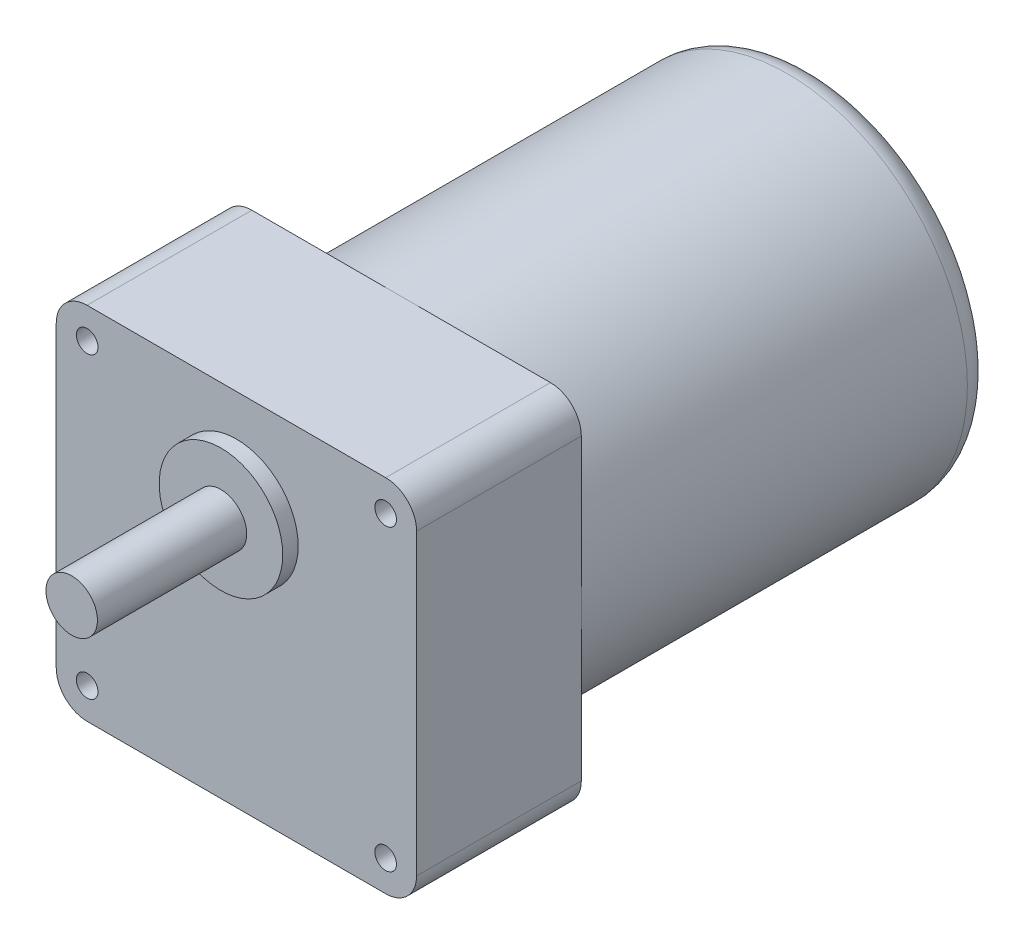
SolidWorks part; units mm, degrees
material "普通碳钢"
ref_plane "Front" through (0, 0, 0) normal (0, 0, 1) x (1, 0, 0)
ref_plane "Top" through (0, 0, 0) normal (0, 1, 0) x (1, 0, 0)
ref_plane "Right" through (0, 0, 0) normal (1, 0, 0) x (0, 0, -1)
sketch "草图1" plane through (0, 0, 0) normal (0, 0, 1) x (1, 0, 0)
  line L1 (-35, 35) -> (35, 35)
  line L2 (-35, 35) -> (-35, -35)
  line L3 (-35, -35) -> (35, -35)
  line L4 (35, 35) -> (35, -35)
  line L5 (-35, 35) -> (35, -35) construction
  line L6 (-35, -35) -> (35, 35) construction
  point P0 (0, 0)
  dimension "D1" = 70
  dimension "D2" = 70
extrude "凸台-拉伸1" add sketch "草图1" along normal blind 32
sketch "草图2" plane through (0, 0, 0) normal (0, 0, -1) x (-1, 0, 0)
  circle A0 centre (0, 0) radius 35
  dimension "D1" = 70
extrude "凸台-拉伸2" add sketch "草图2" along normal blind 80
fillet "圆角1" radius 6 4 edges at (-35, -35, 16) (35, -35, 16) (-35, 35, 16) (35, 35, 16)
fillet "圆角2" radius 5 1 edges at (-35, 0, -80)
sketch "草图3" plane through (0, 0, 32) normal (0, 0, 1) x (1, 0, 0)
  circle A0 centre (0, 15) radius 5
  dimension "D2" = 10
  dimension "D1" = 15
extrude "凸台-拉伸3" add sketch "草图3" along normal blind 32
sketch "草图4" plane through (0, 0, 32) normal (0, 0, 1) x (1, 0, 0)
  line L0 (-28.9914, -28.9914) -> (28.9914, 28.9914) construction
  line L1 (0, 0) -> (0, -46.9372) construction
  line L2 (-28.9914, 28.9914) -> (28.9914, -28.9914) construction
  circle A0 centre (0, 0) radius 41 construction
  dimension "D1" = 82
  dimension "D2" = 90
  dimension "D3" = 45
hole_wizard "M5 螺纹孔1" positions "草图6" profile "草图5" tap size "M5" standard "Gb" end condition through all
sketch "草图6" plane through (0, 0, 32) normal (0, 0, 1) x (1, 0, 0)
  point P0 (-28.9914, 28.9914)
  point P3 (-28.9914, -28.9914)
  point P6 (28.9914, -28.9914)
  point P9 (28.9914, 28.9914)
cosmetic thread "孔螺蚊线1" parameters "D2"=5
cosmetic thread "孔螺蚊线2" parameters "D2"=5
cosmetic thread "孔螺蚊线3" parameters "D2"=5
cosmetic thread "孔螺蚊线4" parameters "D2"=5
sketch "草图5" plane through (-28.9914, 28.9914, 32) normal (1, 0, 0) x (0, -1, 0)
  line L0 (0, 0) -> (0, 112)
  line L1 (0, 112) -> (2.1, 112)
  line L2 (2.1, 112) -> (2.1, 0)
  line L5 (2.1, 0) -> (0, 0)
  line L11 (0, -6.35) -> (0, 107.95) construction
  dimension "通孔螺纹孔钻头直径" = 4.2
  dimension "通孔螺纹孔钻头深度" = 112
sketch "草图7" plane through (0, 0, 32) normal (0, 0, 1) x (1, 0, 0)
  circle A0 centre (0, 15) radius 12
  dimension "D1" = 24
extrude "凸台-拉伸4" add sketch "草图7" along normal blind 3
